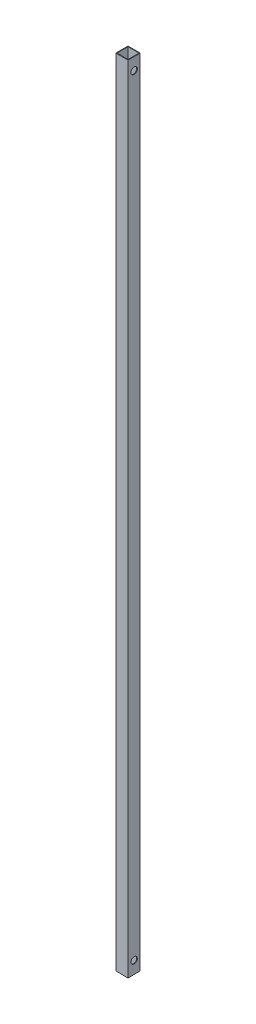
SolidWorks part; units mm, degrees
ref_plane "前视基准面" through (0, 0, 0) normal (0, 0, 1) x (1, 0, 0)
ref_plane "上视基准面" through (0, 0, 0) normal (0, 1, 0) x (1, 0, 0)
ref_plane "右视基准面" through (0, 0, 0) normal (1, 0, 0) x (0, 0, -1)
sketch "草图1" plane through (0, 0, 0) normal (1, 0, 0) x (0, 0, -1)
  line L0 (0, 0) -> (0, 1300)
  dimension "D1" = 1300
other "方通 20 X 20 X 1(1)"
ref_plane "基准面1" through (0, 0, 0) normal (0, 1, 0) x (0, 0, 1)
sketch "Sketch12" plane through (0, 0, 0) normal (0, 1, 0) x (0, 0, 1)
  line L1 (-10, -10) -> (10, -10)
  line L2 (-10, -10) -> (-10, 10)
  line L3 (-10, 10) -> (10, 10)
  line L4 (10, -10) -> (10, 10)
  line L5 (-10, -10) -> (10, 10) construction
  line L6 (-10, 10) -> (10, -10) construction
  line L7 (-9, -9) -> (9, -9)
  line L8 (-9, -9) -> (-9, 9)
  line L9 (-9, 9) -> (9, 9)
  line L10 (9, -9) -> (9, 9)
  line L11 (-9, -9) -> (9, 9) construction
  line L12 (-9, 9) -> (9, -9) construction
  point P0 (0, 0)
  point P5 (0, 0)
  point P10 (0, 0)
  dimension "D1" = 1
  dimension "D2" = 20
hole_wizard "Ø10.5 (10.5) 直径孔1" positions "草图5" profile "草图6" hole size "Ø10.5" standard "GB" end condition through all
sketch "草图5" plane through (10, 0, 0) normal (1, 0, 0) x (0, 0, -1)
  line L0 (0, 0) -> (0, 1300) construction
  line L1 (10, 650) -> (147.7334, 650) construction
  line L2 (10, 1300) -> (10, 0) construction
  line L4 (-10, 1300) -> (10, 1300) construction
  point P0 (0, 20)
  point P4 (0, 1280)
  dimension "D1" = 20
sketch "草图6" plane through (10, 20, 0) normal (0, 1, 0) x (0, 0, -1)
  line L0 (0, 0) -> (0, 20)
  line L1 (0, 20) -> (5.25, 20)
  line L2 (5.25, 20) -> (5.25, 0)
  line L5 (5.25, 0) -> (0, 0)
  line L11 (0, -6.35) -> (0, 107.95) construction
  dimension "通孔孔直径" = 10.5
  dimension "通孔孔深度" = 20
